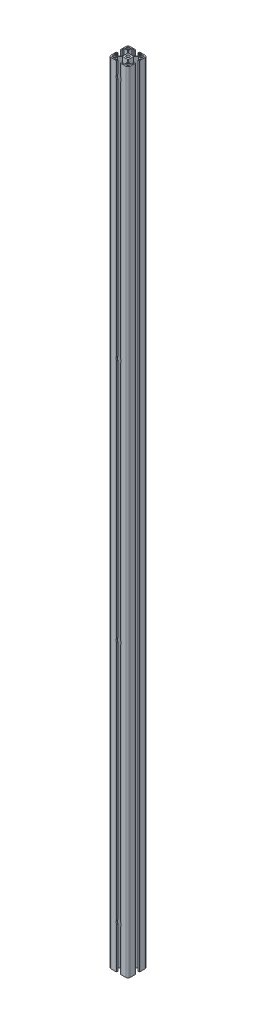
from build123d import *

# Parameters (mm, degrees)
SKETCH1_R                 = 3.4
F_40_X_40L_X_R4_5_1_DEPTH = 1650
HOLE_WIZARD_1_D           = 6.6
HOLE_WIZARD_1_CBORE_D     = 11
HOLE_WIZARD_1_CBORE_DEPTH = 6.8
PATTERN_LINEAR_1_COUNT    = 4
PATTERN_LINEAR_1_PITCH    = 510


with BuildPart() as part:
    # Sketch1 → 铝型材 40 X 40L X R4.5(1) (new body)
    with BuildSketch(Plane.ZX):
        with BuildLine():
            Line((-5.1, 20), (-5.1, 19.5))
            Line((-5.1, 19.5), (-4.1, 19.5))
            Line((-4.1, 19.5), (-4.1, 17))
            Line((-4.1, 17), (-6.1, 17))
            Line((-6.1, 17), (-6.1, 18.5))
            Line((-6.1, 18.5), (-10.3, 18.5))
            Line((-10.3, 18.5), (-10.3, 11.3))
            Line((-10.3, 11.3), (-5, 6))
            Line((-5, 6), (5, 6))
            Line((5, 6), (10.3, 11.3))
            Line((10.3, 11.3), (10.3, 18.5))
            Line((10.3, 18.5), (6.1, 18.5))
            Line((6.1, 18.5), (6.1, 17))
            Line((6.1, 17), (4.1, 17))
            Line((4.1, 17), (4.1, 19.5))
            Line((4.1, 19.5), (5.1, 19.5))
            Line((5.1, 19.5), (5.1, 20))
            Line((5.1, 20), (15.5, 20))
            ThreePointArc((15.5, 20), (18.681980515, 18.681980515), (20, 15.5))
            Line((20, 15.5), (20, 5.1))
            Line((20, 5.1), (19.5, 5.1))
            Line((19.5, 5.1), (19.5, 4.1))
            Line((19.5, 4.1), (17, 4.1))
            Line((17, 4.1), (17, 6.1))
            Line((17, 6.1), (18.5, 6.1))
            Line((18.5, 6.1), (18.5, 10.3))
            Line((18.5, 10.3), (11.3, 10.3))
            Line((11.3, 10.3), (6, 5))
            Line((6, 5), (6, -5))
            Line((6, -5), (11.3, -10.3))
            Line((11.3, -10.3), (18.5, -10.3))
            Line((18.5, -10.3), (18.5, -6.1))
            Line((18.5, -6.1), (17, -6.1))
            Line((17, -6.1), (17, -4.1))
            Line((17, -4.1), (19.5, -4.1))
            Line((19.5, -4.1), (19.5, -5.1))
            Line((19.5, -5.1), (20, -5.1))
            Line((20, -5.1), (20, -15.5))
            ThreePointArc((20, -15.5), (18.681980515, -18.681980515), (15.5, -20))
            Line((15.5, -20), (5.1, -20))
            Line((5.1, -20), (5.1, -19.5))
            Line((5.1, -19.5), (4.1, -19.5))
            Line((4.1, -19.5), (4.1, -17))
            Line((4.1, -17), (6.1, -17))
            Line((6.1, -17), (6.1, -18.5))
            Line((6.1, -18.5), (10.3, -18.5))
            Line((10.3, -18.5), (10.3, -11.3))
            Line((10.3, -11.3), (5, -6))
            Line((5, -6), (-5, -6))
            Line((-5, -6), (-10.3, -11.3))
            Line((-10.3, -11.3), (-10.3, -18.5))
            Line((-10.3, -18.5), (-6.1, -18.5))
            Line((-6.1, -18.5), (-6.1, -17))
            Line((-6.1, -17), (-4.1, -17))
            Line((-4.1, -17), (-4.1, -19.5))
            Line((-4.1, -19.5), (-5.1, -19.5))
            Line((-5.1, -19.5), (-5.1, -20))
            Line((-5.1, -20), (-15.5, -20))
            ThreePointArc((-15.5, -20), (-18.681980515, -18.681980515), (-20, -15.5))
            Line((-20, -15.5), (-20, -5.1))
            Line((-20, -5.1), (-19.5, -5.1))
            Line((-19.5, -5.1), (-19.5, -4.1))
            Line((-19.5, -4.1), (-17, -4.1))
            Line((-17, -4.1), (-17, -6.1))
            Line((-17, -6.1), (-18.5, -6.1))
            Line((-18.5, -6.1), (-18.5, -10.3))
            Line((-18.5, -10.3), (-11.3, -10.3))
            Line((-11.3, -10.3), (-6, -5))
            Line((-6, -5), (-6, 5))
            Line((-6, 5), (-11.3, 10.3))
            Line((-11.3, 10.3), (-18.5, 10.3))
            Line((-18.5, 10.3), (-18.5, 6.1))
            Line((-18.5, 6.1), (-17, 6.1))
            Line((-17, 6.1), (-17, 4.1))
            Line((-17, 4.1), (-19.5, 4.1))
            Line((-19.5, 4.1), (-19.5, 5.1))
            Line((-19.5, 5.1), (-20, 5.1))
            Line((-20, 5.1), (-20, 15.5))
            ThreePointArc((-20, 15.5), (-18.681980515, 18.681980515), (-15.5, 20))
            Line((-15.5, 20), (-5.1, 20))
        make_face()
        Circle(SKETCH1_R, mode=Mode.SUBTRACT)
        with BuildLine():
            Line((11.8, 17.5), (15, 17.5))
            ThreePointArc((15, 17.5), (16.767766953, 16.767766953), (17.5, 15))
            Line((17.5, 15), (17.5, 11.8))
            Line((17.5, 11.8), (11.8, 11.8))
            Line((11.8, 11.8), (11.8, 17.5))
        make_face(mode=Mode.SUBTRACT)
        with BuildLine():
            Line((-15, 17.5), (-11.8, 17.5))
            Line((-11.8, 17.5), (-11.8, 11.8))
            Line((-11.8, 11.8), (-17.5, 11.8))
            Line((-17.5, 11.8), (-17.5, 15))
            ThreePointArc((-17.5, 15), (-16.767766953, 16.767766953), (-15, 17.5))
        make_face(mode=Mode.SUBTRACT)
        with BuildLine():
            Line((-17.5, -11.8), (-11.8, -11.8))
            Line((-11.8, -11.8), (-11.8, -17.5))
            Line((-11.8, -17.5), (-15, -17.5))
            ThreePointArc((-15, -17.5), (-16.767766953, -16.767766953), (-17.5, -15))
            Line((-17.5, -15), (-17.5, -11.8))
        make_face(mode=Mode.SUBTRACT)
        with BuildLine():
            Line((11.8, -11.8), (17.5, -11.8))
            Line((17.5, -11.8), (17.5, -15))
            ThreePointArc((17.5, -15), (16.767766953, -16.767766953), (15, -17.5))
            Line((15, -17.5), (11.8, -17.5))
            Line((11.8, -17.5), (11.8, -11.8))
        make_face(mode=Mode.SUBTRACT)
    extrude(amount=F_40_X_40L_X_R4_5_1_DEPTH)

    # 打孔尺寸(%根据)内六角圆柱头螺钉的类型1 (through all)
    with Locations(Plane.XY.offset(20)):
        with Locations((0, 1620)):
            hole_wizard_1 = CounterBoreHole(HOLE_WIZARD_1_D / 2, HOLE_WIZARD_1_CBORE_D / 2, HOLE_WIZARD_1_CBORE_DEPTH)

    # 阵列(线性)1: 打孔尺寸(%根据)内六角圆柱头螺钉的类型1 ×4
    with Locations(*[(0, -i * PATTERN_LINEAR_1_PITCH, 0) for i in range(1, PATTERN_LINEAR_1_COUNT)]):
        add(hole_wizard_1, mode=Mode.SUBTRACT)


solid = part.part
